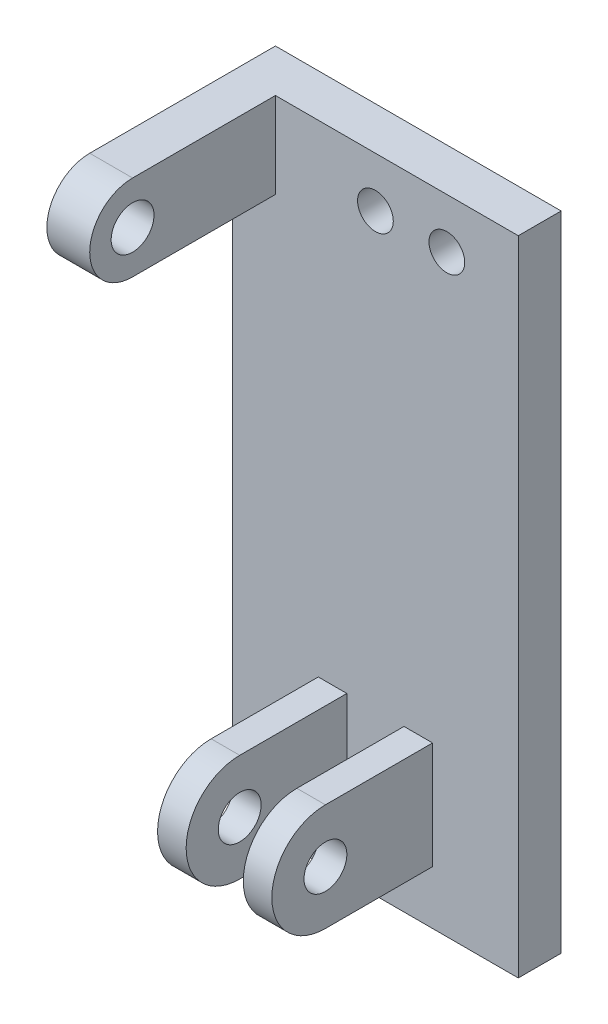
SolidWorks part; units mm, degrees
ref_plane "Front Plane" through (0, 0, 0) normal (0, 0, 1) x (1, 0, 0)
ref_plane "Top Plane" through (0, 0, 0) normal (0, 1, 0) x (1, 0, 0)
ref_plane "Right Plane" through (0, 0, 0) normal (1, 0, 0) x (0, 0, -1)
sketch "Sketch1" plane through (0, 0, 0) normal (0, 0, 1) x (1, 0, 0)
  line L1 (-20, 45) -> (20, 45)
  line L2 (-20, 45) -> (-20, -45)
  line L3 (-20, -45) -> (20, -45)
  line L4 (20, 45) -> (20, -45)
  line L5 (-20, 45) -> (20, -45) construction
  line L6 (-20, -45) -> (20, 45) construction
  point P0 (0, 0)
  dimension "D1" = 90
  dimension "D2" = 40
extrude "Boss-Extrude1" add sketch "Sketch1" along normal blind 6
sketch "Sketch2" plane through (0, 0, 6) normal (0, 0, 1) x (1, 0, 0)
  circle A0 centre (0, 38) radius 2.5
  circle A1 centre (10, 38) radius 2.5
  dimension "D1" = 38
  dimension "D2" = 5
  dimension "D3" = 10
extrude "Cut-Extrude1" cut sketch "Sketch2" against normal blind 6
sketch "Sketch3" plane through (-20, 0, 0) normal (-1, 0, 0) x (0, 0, 1)
  line L0 (6, 45) -> (0, 45) construction
  line L1 (6, 45) -> (6, -45) construction
  line L2 (26, 45) -> (6, 45)
  line L3 (6, 45) -> (6, 33)
  line L4 (6, 33) -> (26, 33)
  circle A0 centre (26, 39) radius 3
  arc A1 (26, 33) -> (26, 45) centre (26, 39) ccw
  dimension "D2" = 6
  dimension "D3" = 12
  dimension "D1" = 20
extrude "Boss-Extrude2" add sketch "Sketch3" against normal blind 6
sketch "Sketch4" plane through (0, 0, 0) normal (1, 0, 0) x (0, 0, -1)
  line L0 (-6, -45) -> (-6, 45) construction
  line L1 (-21, -22.5) -> (-6, -22.5)
  line L2 (-6, -22.5) -> (-6, -37.5)
  line L3 (-6, -37.5) -> (-21, -37.5)
  circle A0 centre (-21, -30) radius 3
  arc A1 (-21, -22.5) -> (-21, -37.5) centre (-21, -30) ccw
  dimension "D1" = 6
  dimension "D2" = 15
  dimension "D3" = 15
  dimension "D4" = 30
extrude "Boss-Extrude3" add sketch "Sketch4" along normal blind 4 from offset 4
mirror "Mirror1" about plane through (0, 0, 0) normal (1, 0, 0) of "Boss-Extrude3"
